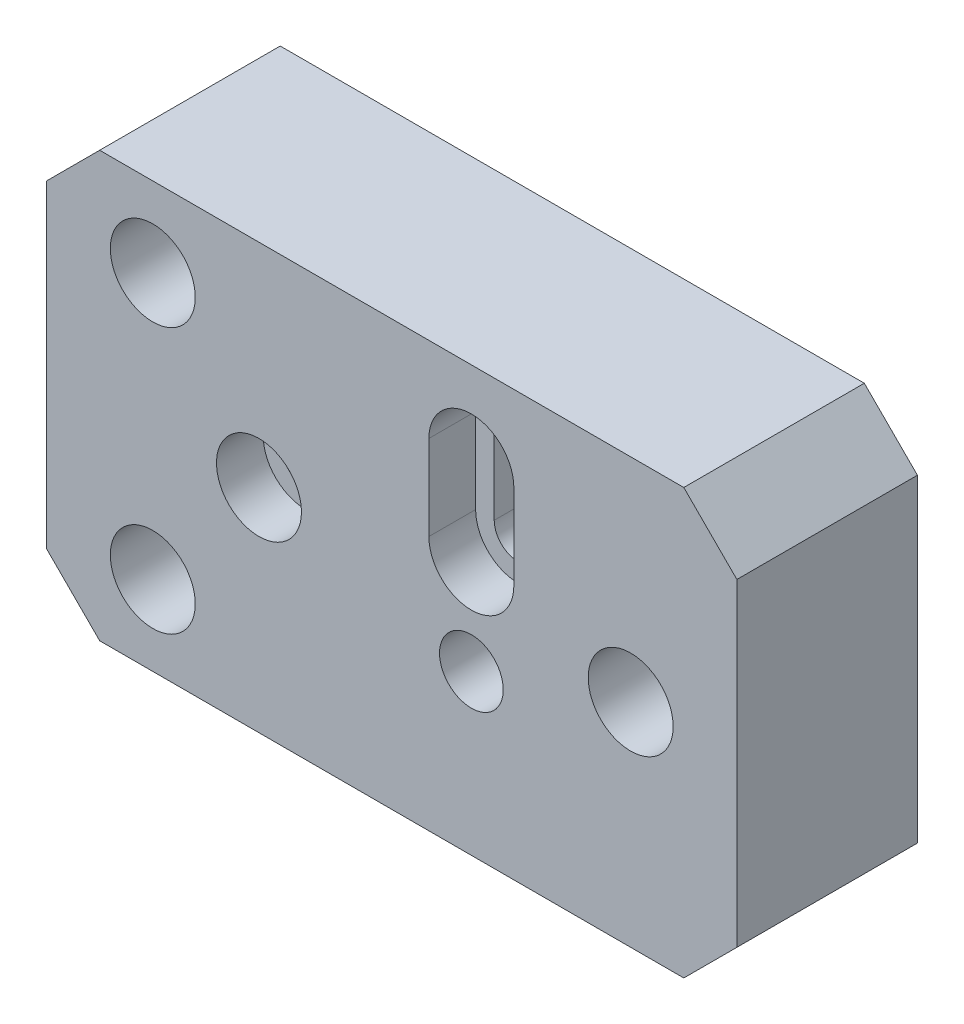
SolidWorks part; units mm, degrees
material "SUS304"
ref_plane "前视基准面" through (0, 0, 0) normal (0, 0, 1) x (1, 0, 0)
ref_plane "上视基准面" through (0, 0, 0) normal (0, 1, 0) x (1, 0, 0)
ref_plane "右视基准面" through (0, 0, 0) normal (1, 0, 0) x (0, 0, -1)
sketch "草图1" plane through (0, 0, 0) normal (0, 0, 1) x (1, 0, 0)
  line L1 (-32.5, -20) -> (32.5, -20)
  line L2 (-32.5, -20) -> (-32.5, 20)
  line L3 (-32.5, 20) -> (32.5, 20)
  line L4 (32.5, -20) -> (32.5, 20)
  line L5 (-32.5, -20) -> (32.5, 20) construction
  line L6 (-32.5, 20) -> (32.5, -20) construction
  point P0 (0, 0)
  dimension "D1" = 65
  dimension "D2" = 40
extrude "凸台-拉伸1" add sketch "草图1" along normal mid plane 17
hole_wizard "Ø8.0 (8) 直径孔1" positions "草图3" profile "草图2" hole size "Ø8.0" standard "ISO" end condition through all
sketch "草图3" plane through (0, 0, 8.5) normal (0, 0, 1) x (1, 0, 0)
  line L0 (-32.5, 20) -> (-32.5, -20) construction
  line L1 (32.5, 0) -> (-32.5, 0) construction
  line L2 (32.5, -20) -> (32.5, 20) construction
  point P0 (-22.5, 12.5)
  point P2 (-22.5, -12.5)
  point P4 (22.5, 0)
  dimension "D1" = 10
  dimension "D2" = 25
  dimension "D3" = 45
sketch "草图2" plane through (-22.5, 12.5, 8.5) normal (1, 0, 0) x (0, -1, 0)
  line L0 (0, 0) -> (0, 17)
  line L1 (0, 17) -> (4, 17)
  line L2 (4, 17) -> (4, 0)
  line L5 (4, 0) -> (0, 0)
  line L11 (0, -6.35) -> (0, 107.95) construction
  dimension "通孔孔直径" = 8
  dimension "通孔孔深度" = 17
sketch "草图4" plane through (0, 0, -8.5) normal (0, 0, -1) x (-1, 0, 0)
  line L0 (32.5, 20) -> (32.5, -20) construction
  circle A0 centre (12.5, 0) radius 6
  dimension "D1" = 12
  dimension "D2" = 20
extrude "切除-拉伸1" cut sketch "草图4" against normal blind 9.5
hole_wizard "M4 六角凹头螺钉的柱形沉头孔1" positions "草图6" profile "草图5" counterbore size "M4" standard "ISO" end condition through all
sketch "草图6" plane through (0, 0, 8.5) normal (0, 0, 1) x (1, 0, 0)
  point P0 (-12.5, 0)
sketch "草图5" plane through (-12.5, 0, 8.5) normal (1, 0, 0) x (0, -1, 0)
  line L0 (0, 0) -> (0, 17)
  line L1 (0, 17) -> (2.25, 17)
  line L3 (2.25, 17) -> (2.25, 4.4)
  line L4 (2.25, 4.4) -> (4, 4.4)
  line L5 (4, 4.4) -> (4, 0)
  line L7 (4, 0) -> (0, 0)
  line L11 (0, -6.35) -> (0, 107.95) construction
  dimension "通孔孔直径" = 4.5
  dimension "通孔孔深度" = 17
  dimension "柱形沉头孔直径" = 8
  dimension "柱形沉头孔深度" = 4.4
hole_wizard "Ø6.0 (6) 直径孔1" positions "草图8" profile "草图7" hole size "Ø6.0" standard "ISO" end condition through all
sketch "草图8" plane through (0, 0, -8.5) normal (0, 0, -1) x (-1, 0, 0)
  line L0 (32.5, -20) -> (-32.5, -20) construction
  circle A0 centre (12.5, 0) radius 2.25 construction
  point P0 (-7.5, -5)
  dimension "D1" = 20
  dimension "D2" = 15
sketch "草图7" plane through (7.5, -5, -8.5) normal (1, 0, 0) x (0, 1, 0)
  line L0 (0, 0) -> (0, 17)
  line L1 (0, 17) -> (3, 17)
  line L2 (3, 17) -> (3, 0)
  line L5 (3, 0) -> (0, 0)
  line L11 (0, -6.35) -> (0, 107.95) construction
  dimension "通孔孔直径" = 6
  dimension "通孔孔深度" = 17
sketch "草图9" plane through (0, 0, -8.5) normal (0, 0, -1) x (-1, 0, 0)
  line L0 (-7.5, 4) -> (-7.5, 12) construction
  line L1 (-11.5, 4) -> (-11.5, 12)
  line L2 (-3.5, 4) -> (-3.5, 12)
  line L3 (-32.5, 20) -> (32.5, 20) construction
  arc A0 (-11.5, 4) -> (-3.5, 4) centre (-7.5, 4) ccw
  arc A1 (-3.5, 12) -> (-11.5, 12) centre (-7.5, 12) ccw
  circle A2 centre (12.5, 0) radius 6 construction
  circle A3 centre (-7.5, -5) radius 3 construction
  point P2 (-7.5, 8)
  dimension "D1" = 4
  dimension "D2" = 20
  dimension "D3" = 9
  dimension "D4" = 8
extrude "切除-拉伸2" cut sketch "草图9" against normal up to surface (9.5 mm away) up to face at (-14.75, 0, 1)
sketch "草图10" plane through (0, 0, 8.5) normal (0, 0, 1) x (1, 0, 0)
  line L0 (7.5, 4) -> (7.5, 12) construction
  line L1 (5.25, 4) -> (5.25, 12)
  line L2 (9.75, 4) -> (9.75, 12)
  arc A0 (5.25, 4) -> (9.75, 4) centre (7.5, 4) ccw
  arc A1 (9.75, 12) -> (5.25, 12) centre (7.5, 12) ccw
  point P4 (7.5, 8)
  dimension "D1" = 2.25
extrude "切除-拉伸3" cut sketch "草图10" against normal through all
sketch "草图11" plane through (0, 0, 8.5) normal (0, 0, 1) x (1, 0, 0)
  line L0 (7.5, 4) -> (7.5, 12) construction
  line L1 (3.5, 4) -> (3.5, 12)
  line L2 (11.5, 4) -> (11.5, 12)
  arc A0 (3.5, 4) -> (11.5, 4) centre (7.5, 4) ccw
  arc A1 (11.5, 12) -> (3.5, 12) centre (7.5, 12) ccw
  point P4 (7.5, 8)
  dimension "D1" = 4
extrude "切除-拉伸4" cut sketch "草图11" against normal up to surface (4.4 mm away) up to face at (-10.25, 0, 4.1)
chamfer "倒角1" distance 5 angle 45 4 edges at (-32.5, -20, 0) (-32.5, 20, 0) (32.5, 20, 0) (32.5, -20, 0)
